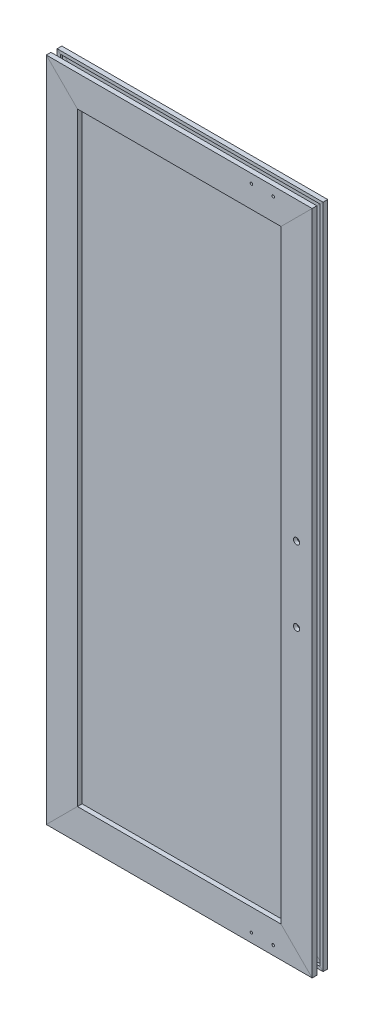
SolidWorks part; units mm, degrees
material "铝型材"
ref_plane "前视基准面" through (0, 0, 0) normal (0, 0, 1) x (1, 0, 0)
ref_plane "上视基准面" through (0, 0, 0) normal (0, 1, 0) x (1, 0, 0)
ref_plane "右视基准面" through (0, 0, 0) normal (1, 0, 0) x (0, 0, -1)
sketch "草图13" plane through (0, 0, 0) normal (0, 0, 1) x (1, 0, 0)
  line L1 (-150.75, -408) -> (150.75, -408)
  line L2 (-150.75, -408) -> (-150.75, 408)
  line L3 (-150.75, 408) -> (150.75, 408)
  line L4 (150.75, -408) -> (150.75, 408)
  line L5 (-150.75, -408) -> (150.75, 408) construction
  line L6 (-150.75, 408) -> (150.75, -408) construction
  point P0 (0, 0)
  dimension "D1" = 301.5
  dimension "D2" = 816
other "铝型材 2040A(1)"
ref_plane "基准面3" through (-150.75, 408, 0) normal (1, 0, 0) x (0, 1, 0)
sketch "草图19" plane through (-150.75, 408, 0) normal (1, 0, 0) x (0, 1, 0)
  line L0 (9, 4) -> (6, 4)
  line L1 (9, 4) -> (9, 7)
  line L2 (6, -4) -> (6, 4)
  line L3 (16, 7) -> (9, 7)
  line L4 (9, -4) -> (6, -4)
  line L5 (16, 4) -> (16, 7)
  line L6 (9, -7) -> (9, -4)
  line L7 (20, 4) -> (16, 4)
  line L8 (16, -7) -> (9, -7)
  line L9 (20, 10) -> (20, 4)
  line L10 (16, -7) -> (16, -4)
  line L11 (-20, 10) -> (20, 10)
  line L12 (20, -4) -> (16, -4)
  line L13 (-20, 4) -> (-20, 10)
  line L14 (20, -4) -> (20, -10)
  line L15 (-20, 4) -> (-16, 4)
  line L16 (20, -10) -> (-20, -10)
  line L17 (-16, 4) -> (-16, 7)
  line L18 (-20, -10) -> (-20, -4)
  line L19 (-16, 7) -> (-9, 7)
  line L20 (-20, -4) -> (-16, -4)
  line L21 (-9, 4) -> (-9, 7)
  line L22 (-16, -7) -> (-16, -4)
  line L23 (-9, 4) -> (-6, 4)
  line L24 (-16, -7) -> (-9, -7)
  line L25 (-6, -4) -> (-6, 4)
  line L26 (-9, -7) -> (-9, -4)
  line L27 (-9, -4) -> (-6, -4)
  circle A0 centre (0, 0) radius 3.25
  point P0 (0, 0)
sketch "草图14" plane through (0, 0, 0) normal (0, 0, 1) x (1, 0, 0)
  line L0 (156.75, 414) -> (159.75, 417) construction
  line L1 (-144.25, -401.5) -> (144.25, -401.5)
  line L2 (-144.25, -401.5) -> (-144.25, 401.5)
  line L3 (-144.25, 401.5) -> (144.25, 401.5)
  line L4 (144.25, -401.5) -> (144.25, 401.5)
  line L5 (-144.25, -401.5) -> (144.25, 401.5) construction
  line L6 (-144.25, 401.5) -> (144.25, -401.5) construction
  line L8 (130.75, 388) -> (-130.75, 388) construction
  point P0 (0, 0)
  dimension "D1" = 13.5
extrude "凸台-拉伸1" add sketch "草图14" along normal mid plane 4 separate body
hole_wizard "M4 螺纹孔2" positions "草图24" profile "草图25" tap size "M4" standard "GB"
sketch "草图24" plane through (0, 0, 10) normal (0, 0, -1) x (-1, 0, 0)
  line L0 (-120.75, 416.5) -> (-92.75, 416.5) construction
  line L7 (0, 0) -> (81.0682, 0) construction
  line L10 (-170.75, 428) -> (170.75, 428) construction
  line L11 (-170.75, -428) -> (-170.75, 428) construction
  point P0 (-120.75, 416.5)
  point P2 (-92.75, 416.5)
  point P29 (-92.75, -416.5)
  point P30 (-120.75, -416.5)
  dimension "D1" = 28
  dimension "D2" = 11.5
  dimension "D3" = 50
cosmetic thread "孔螺蚊线3"
cosmetic thread "孔螺蚊线4"
cosmetic thread "孔螺蚊线9"
cosmetic thread "孔螺蚊线10"
sketch "草图25" plane through (120.75, 416.5, 10) normal (1, 0, 0) x (0, -1, 0)
  line L0 (0, 0) -> (0, 11.0914)
  line L1 (0, 11.0914) -> (1.65, 10.1)
  line L2 (1.65, 10.1) -> (1.65, 0)
  line L5 (1.65, 0) -> (0, 0)
  line L10 (0, 11.0914) -> (-1.65, 10.1) construction
  line L11 (0, -6.35) -> (0, 107.95) construction
  dimension "螺纹孔钻头直径" = 3.3
  dimension "螺纹孔钻头深度" = 10.1
  dimension "导头角度" = 118
hole_wizard "打孔尺寸(%根据)开槽圆柱头螺钉的类型1" positions "草图26" profile "草图27" counterbore size "M4" standard "GB" end condition through all
sketch "草图26" plane through (0, 0, 10) normal (0, 0, 1) x (1, 0, 0)
  line L0 (0, 0) -> (50000, 0) construction
  line L1 (150.75, 424) -> (150.75, -49576) construction
  line L2 (170.75, 428) -> (130.75, 388) construction
  point P0 (150.75, 48)
  point P2 (150.75, -48)
  point P14 (150.75, 408)
  dimension "D1" = 96
sketch "草图27" plane through (150.75, 48, 10) normal (1, 0, 0) x (0, -1, 0)
  line L0 (0, 0) -> (0, 20)
  line L1 (0, 20) -> (2.25, 20)
  line L3 (2.25, 20) -> (2.25, 4.6)
  line L4 (2.25, 4.6) -> (4, 4.6)
  line L5 (4, 4.6) -> (4, 0)
  line L7 (4, 0) -> (0, 0)
  line L11 (0, -6.35) -> (0, 107.95) construction
  dimension "通孔孔直径" = 4.5
  dimension "通孔孔深度" = 20
  dimension "柱形沉头孔直径" = 8
  dimension "柱形沉头孔深度" = 4.6
hole_wizard "M6 螺纹孔1" positions "草图28" profile "草图29" tap size "M6" standard "GB"
sketch "草图28" plane through (0, 0, -10) normal (0, 0, -1) x (-1, 0, 0)
  line L0 (0, 0) -> (50000, 0) construction
  line L1 (150.75, 424) -> (150.75, -49576) construction
  line L2 (130.75, 388) -> (170.75, 428) construction
  line L3 (-170.75, 428) -> (170.75, 428) construction
  line L4 (150.75, -469.5) -> (150.75, 49530.5) construction
  point P0 (150.75, 328)
  point P2 (150.75, 291)
  point P12 (150.75, 408)
  point P19 (150.75, -328)
  point P20 (150.75, -291)
  dimension "D1" = 100
  dimension "D2" = 37
sketch "草图29" plane through (-150.75, 328, -10) normal (1, 0, 0) x (0, 1, 0)
  line L0 (0, 0) -> (0, 18.5022)
  line L1 (0, 18.5022) -> (2.5, 17)
  line L2 (2.5, 17) -> (2.5, 0)
  line L5 (2.5, 0) -> (0, 0)
  line L10 (0, 18.5022) -> (-2.5, 17) construction
  line L11 (0, -6.35) -> (0, 107.95) construction
  dimension "螺纹孔钻头直径" = 5
  dimension "螺纹孔钻头深度" = 17
  dimension "导头角度" = 118
cosmetic thread "孔螺蚊线5"
cosmetic thread "孔螺蚊线6"
cosmetic thread "孔螺蚊线7"
cosmetic thread "孔螺蚊线8"
